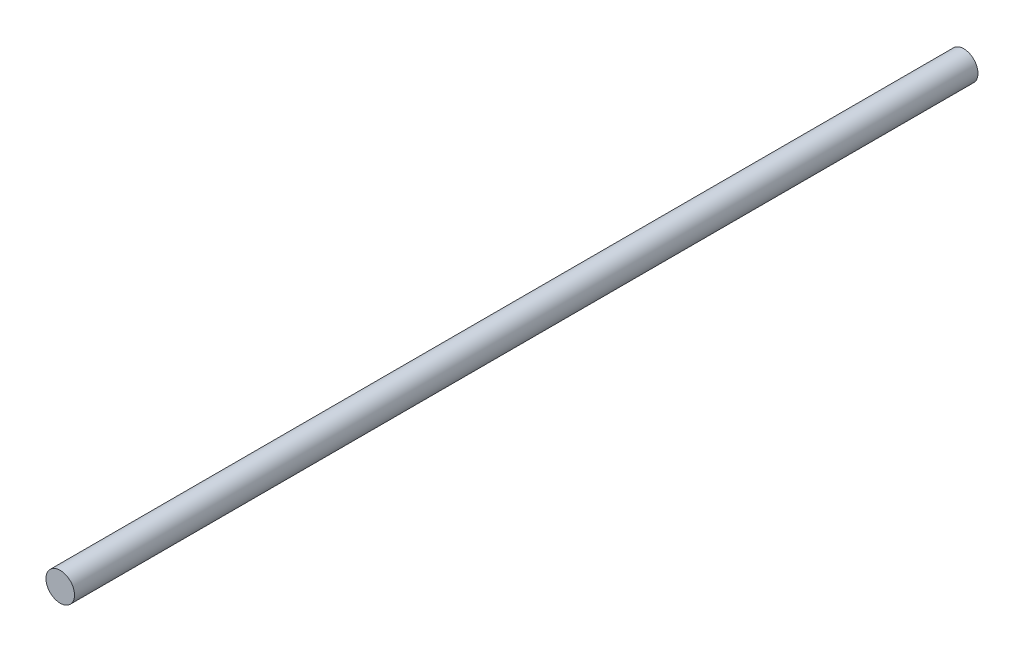
SolidWorks part; units mm, degrees
ref_plane "前视基准面" through (0, 0, 0) normal (0, 0, 1) x (1, 0, 0)
ref_plane "上视基准面" through (0, 0, 0) normal (0, 1, 0) x (1, 0, 0)
ref_plane "右视基准面" through (0, 0, 0) normal (1, 0, 0) x (0, 0, -1)
other "Configuration Table"
sketch "草图1" plane through (0, 0, 0) normal (0, 0, 1) x (1, 0, 0)
  circle A0 centre (0, 0) radius 6
  point P0 (0, 0)
  dimension "D1" = 12
extrude "凸台-拉伸1" add sketch "草图1" against normal mid plane 380
